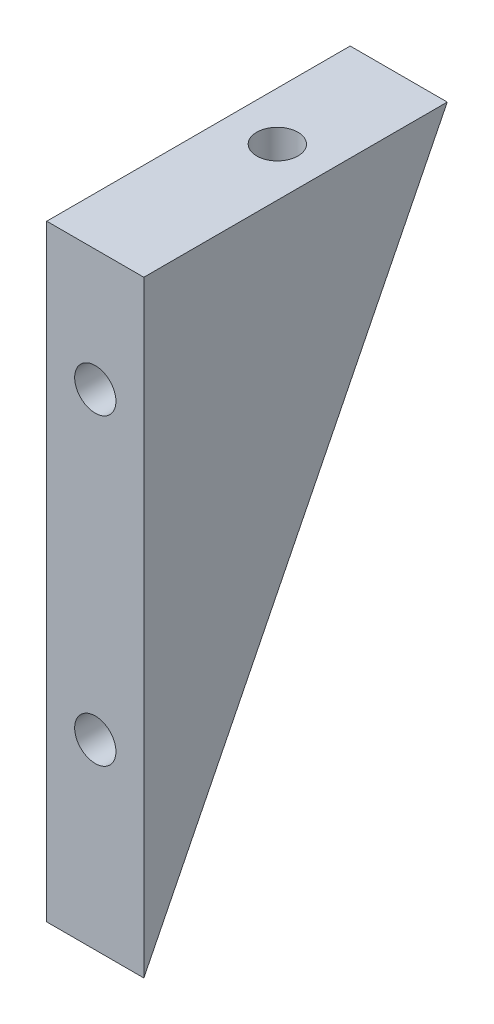
SolidWorks part; units mm, degrees
ref_plane "前视基准面" through (0, 0, 0) normal (0, 0, 1) x (1, 0, 0)
ref_plane "上视基准面" through (0, 0, 0) normal (0, 1, 0) x (1, 0, 0)
ref_plane "右视基准面" through (0, 0, 0) normal (1, 0, 0) x (0, 0, -1)
sketch "草图1" plane through (0, 0, 0) normal (1, 0, 0) x (0, 0, -1)
  line L0 (0, 0) -> (50, 0)
  line L1 (50, 0) -> (0, -100)
  line L2 (0, -100) -> (0, 0)
  dimension "D1" = 50
  dimension "D2" = 100
extrude "凸台-拉伸1" add sketch "草图1" along normal blind 16
hole_wizard "M8 螺纹孔1" positions "草图2" profile "草图3" tap size "M8" standard "GB"
sketch "草图2" plane through (0, 0, 0) normal (0, 1, 0) x (1, 0, 0)
  line L0 (8, 0) -> (8, 49.053) construction
  line L1 (16, 0) -> (0, 0) construction
  point P0 (8, 30)
  dimension "D1" = 30
sketch "草图3" plane through (8, 0, -30) normal (1, 0, 0) x (0, 0, 1)
  line L0 (0, 0) -> (0, 31.2929)
  line L1 (0, 31.2929) -> (3.4, 29.25)
  line L2 (3.4, 29.25) -> (3.4, 0)
  line L5 (3.4, 0) -> (0, 0)
  line L10 (0, 31.2929) -> (-3.4, 29.25) construction
  line L11 (0, -6.35) -> (0, 107.95) construction
  dimension "螺纹孔钻头直径" = 6.8
  dimension "螺纹孔钻头深度" = 29.25
  dimension "导头角度" = 118
cosmetic thread "孔螺蚊线1"
hole_wizard "M8 螺纹孔2" positions "草图4" profile "草图5" tap size "M8" standard "GB"
sketch "草图4" plane through (0, 0, 0) normal (0, 0, 1) x (1, 0, 0)
  line L0 (8, -100) -> (8, -35.6503) construction
  line L1 (16, -100) -> (0, -100) construction
  line L3 (16, 0) -> (0, 0) construction
  point P0 (8, -20)
  point P2 (8, -70)
  dimension "D1" = 20
  dimension "D2" = 50
sketch "草图5" plane through (8, -20, 0) normal (1, 0, 0) x (0, -1, 0)
  line L0 (0, 0) -> (0, 31.2929)
  line L1 (0, 31.2929) -> (3.4, 29.25)
  line L2 (3.4, 29.25) -> (3.4, 0)
  line L5 (3.4, 0) -> (0, 0)
  line L10 (0, 31.2929) -> (-3.4, 29.25) construction
  line L11 (0, -6.35) -> (0, 107.95) construction
  dimension "螺纹孔钻头直径" = 6.8
  dimension "螺纹孔钻头深度" = 29.25
  dimension "导头角度" = 118
cosmetic thread "孔螺蚊线2"
cosmetic thread "孔螺蚊线3"
